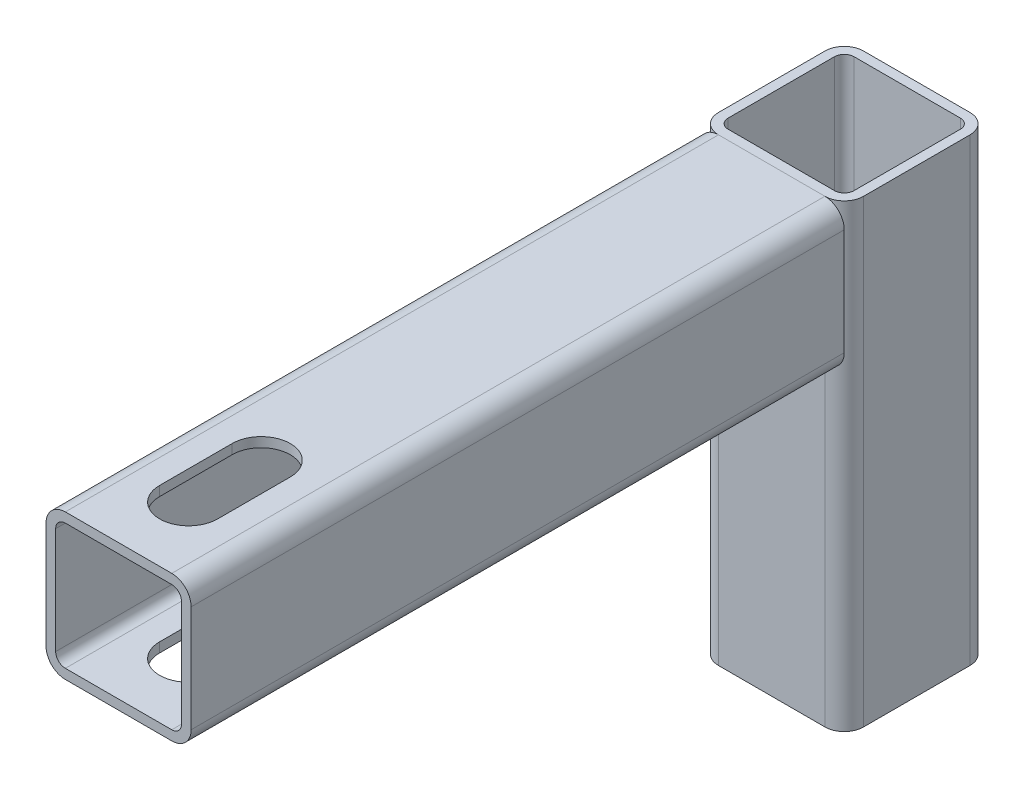
from build123d import *

# Parameters (mm, degrees)
GB_6728_1986_030_X_30_X_2_1_DEPTH        = 95
GB_6728_1986_030_X_30_X_2_1_2_DEPTH      = 150
GB_6728_1986_030_X_30_X_2_1_2_DEPTH_BACK = 1
CUT_EXTRUDE_1_DEPTH                      = 67


with BuildPart() as part:
    # Sketch13 on segment 1 (carried to segment 1) → Gb／6728-1986方形空心型钢 030 X 30 X 2(1) (new body)
    with BuildSketch(Plane.ZX):
        with BuildLine():
            Line((-11, -15), (11, -15))
            ThreePointArc((11, -15), (13.828427125, -13.828427125), (15, -11))
            Line((15, -11), (15, 11))
            ThreePointArc((15, 11), (13.828427125, 13.828427125), (11, 15))
            Line((11, 15), (-11, 15))
            ThreePointArc((-11, 15), (-13.828427125, 13.828427125), (-15, 11))
            Line((-15, 11), (-15, -11))
            ThreePointArc((-15, -11), (-13.828427125, -13.828427125), (-11, -15))
        make_face()
        with BuildLine():
            Line((-11, -13), (11, -13))
            ThreePointArc((11, -13), (12.414213562, -12.414213562), (13, -11))
            Line((13, -11), (13, 11))
            ThreePointArc((13, 11), (12.414213562, 12.414213562), (11, 13))
            Line((11, 13), (-11, 13))
            ThreePointArc((-11, 13), (-12.414213562, 12.414213562), (-13, 11))
            Line((-13, 11), (-13, -11))
            ThreePointArc((-13, -11), (-12.414213562, -12.414213562), (-11, -13))
        make_face(mode=Mode.SUBTRACT)
    extrude(amount=GB_6728_1986_030_X_30_X_2_1_DEPTH)


with BuildPart() as body_2:
    # Sketch13 → Gb_6728-1986_ 030 X 30 X 2_1 2 (new, two sides: drawn at the far end of the back side and taken through both)
    with BuildSketch(Plane(origin=(0, 80, 0), x_dir=(0, -1, 0), z_dir=(0, 0, 1)).offset(-GB_6728_1986_030_X_30_X_2_1_2_DEPTH_BACK)):
        with BuildLine():
            Line((-11, -15), (11, -15))
            ThreePointArc((11, -15), (13.828427125, -13.828427125), (15, -11))
            Line((15, -11), (15, 11))
            ThreePointArc((15, 11), (13.828427125, 13.828427125), (11, 15))
            Line((11, 15), (-11, 15))
            ThreePointArc((-11, 15), (-13.828427125, 13.828427125), (-15, 11))
            Line((-15, 11), (-15, -11))
            ThreePointArc((-15, -11), (-13.828427125, -13.828427125), (-11, -15))
        make_face()
        with BuildLine():
            Line((-11, -13), (11, -13))
            ThreePointArc((11, -13), (12.414213562, -12.414213562), (13, -11))
            Line((13, -11), (13, 11))
            ThreePointArc((13, 11), (12.414213562, 12.414213562), (11, 13))
            Line((11, 13), (-11, 13))
            ThreePointArc((-11, 13), (-12.414213562, 12.414213562), (-13, 11))
            Line((-13, 11), (-13, -11))
            ThreePointArc((-13, -11), (-12.414213562, -12.414213562), (-11, -13))
        make_face(mode=Mode.SUBTRACT)
    extrude(amount=GB_6728_1986_030_X_30_X_2_1_2_DEPTH + GB_6728_1986_030_X_30_X_2_1_2_DEPTH_BACK)

    # Gb_6728-1986_ 030 X 30 X 2_1 2 end butt
    split(bisect_by=Plane(origin=(0, 80, 15), x_dir=(0, -1, 0), z_dir=(0, 0, 1)), keep=Keep.TOP)

    # 草图6 → 切除-拉伸1 (cut)
    with BuildSketch(Plane(origin=(0, 95, 0), x_dir=(1, 0, 0), z_dir=(0, 1, 0))):
        with BuildLine():
            Line((-6, -135.514198409), (-6, -120.514198409))
            ThreePointArc((-6, -120.514198409), (0, -114.514198409), (6, -120.514198409))
            Line((6, -120.514198409), (6, -135.514198409))
            ThreePointArc((6, -135.514198409), (0, -141.514198409), (-6, -135.514198409))
        make_face()
    extrude(amount=-CUT_EXTRUDE_1_DEPTH, mode=Mode.SUBTRACT)


solid = Compound([part.part, body_2.part])
